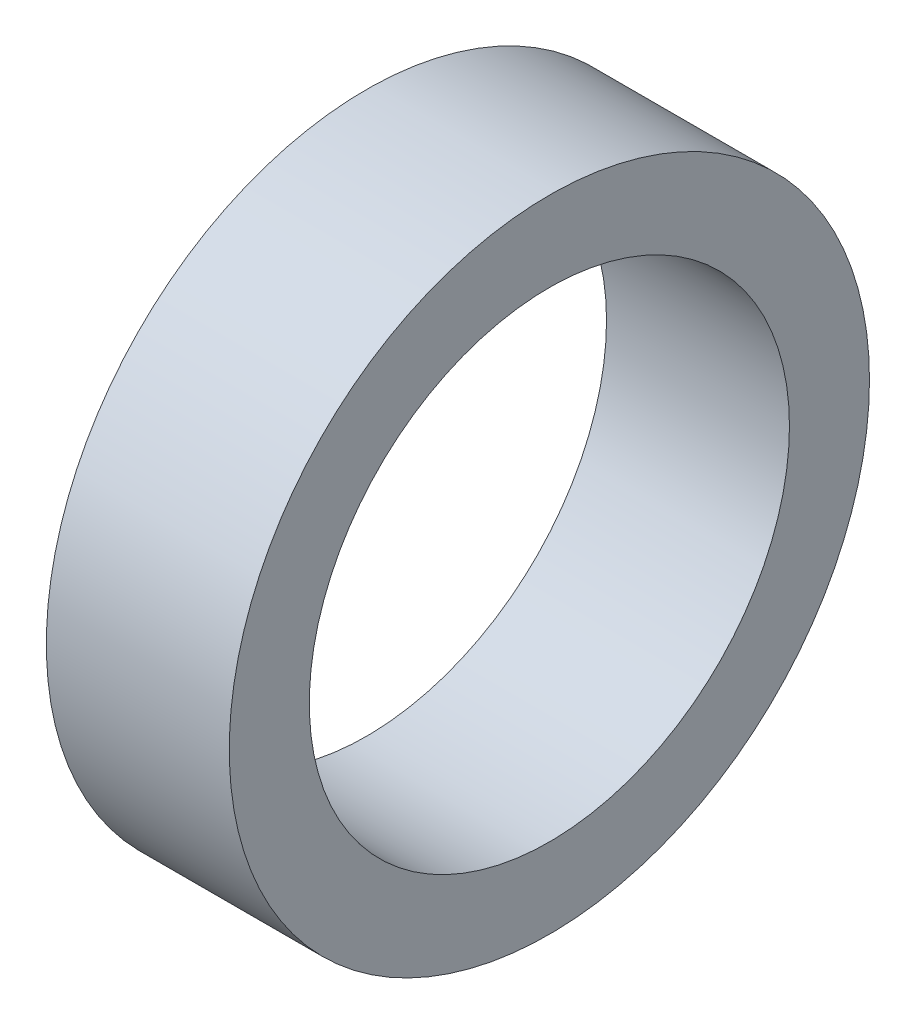
SolidWorks part; units mm, degrees
material "Q235-A"
ref_plane "Front" through (0, 0, 0) normal (0, 0, 1) x (1, 0, 0)
ref_plane "Top" through (0, 0, 0) normal (0, 1, 0) x (1, 0, 0)
ref_plane "Right" through (0, 0, 0) normal (1, 0, 0) x (0, 0, -1)
sketch "草图1" plane through (0, 0, 0) normal (1, 0, 0) x (0, 0, -1)
  circle A0 centre (0, 0) radius 7
  circle A1 centre (0, 0) radius 5.25
  dimension "D1" = 10.5
  dimension "D2" = 14
extrude "凸台-拉伸1" add sketch "草图1" along normal blind 4
